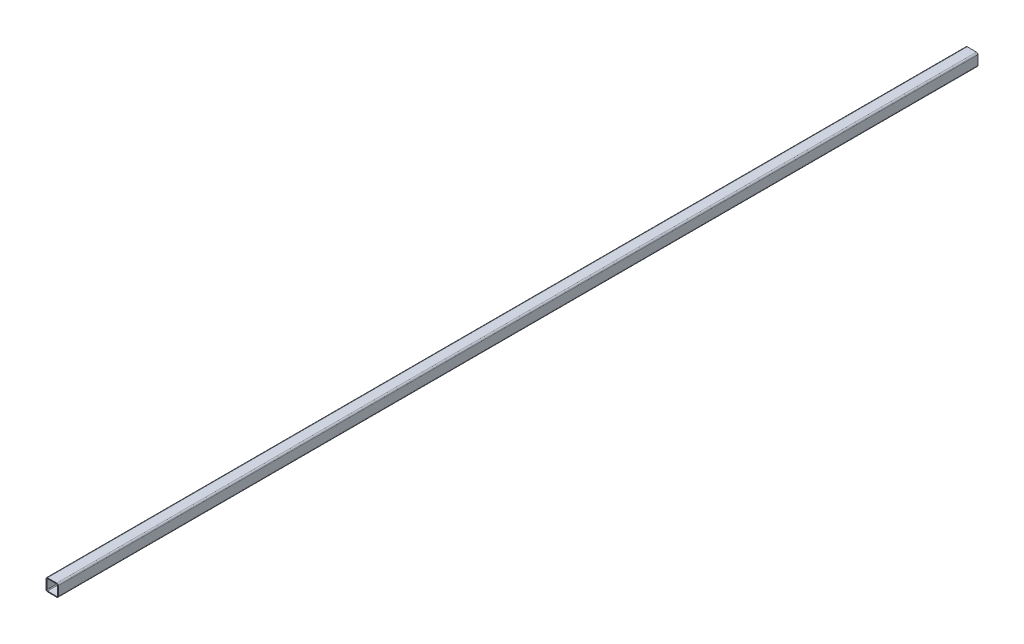
from build123d import *

# Parameters (mm, degrees)
BOSS_EXTRUDE_1_DEPTH = 2400


with BuildPart() as part:
    # Sketch 1 → Boss-Extrude 1 (new, symmetric)
    with BuildSketch(Plane.XY):
        with BuildLine():
            Line((0, 32), (-24, 32))
            ThreePointArc((-24, 32), (-29.656854249, 29.656854249), (-32, 24))
            Line((-32, 24), (-32, 0))
            Line((-32, 0), (-32, -24))
            ThreePointArc((-32, -24), (-29.656854249, -29.656854249), (-24, -32))
            Line((-24, -32), (24, -32))
            ThreePointArc((24, -32), (29.656854249, -29.656854249), (32, -24))
            Line((32, -24), (32, 0))
            Line((32, 0), (32, 24))
            ThreePointArc((32, 24), (29.656854249, 29.656854249), (24, 32))
            Line((24, 32), (0, 32))
        make_face()
        with BuildLine():
            Line((0, 28), (-24, 28))
            ThreePointArc((-24, 28), (-26.828427125, 26.828427125), (-28, 24))
            Line((-28, 24), (-28, 0))
            Line((-28, 0), (-28, -24))
            ThreePointArc((-28, -24), (-26.828427125, -26.828427125), (-24, -28))
            Line((-24, -28), (24, -28))
            ThreePointArc((24, -28), (26.828427125, -26.828427125), (28, -24))
            Line((28, -24), (28, 0))
            Line((28, 0), (28, 24))
            ThreePointArc((28, 24), (26.828427125, 26.828427125), (24, 28))
            Line((24, 28), (0, 28))
        make_face(mode=Mode.SUBTRACT)
    extrude(amount=BOSS_EXTRUDE_1_DEPTH, both=True)


solid = part.part
